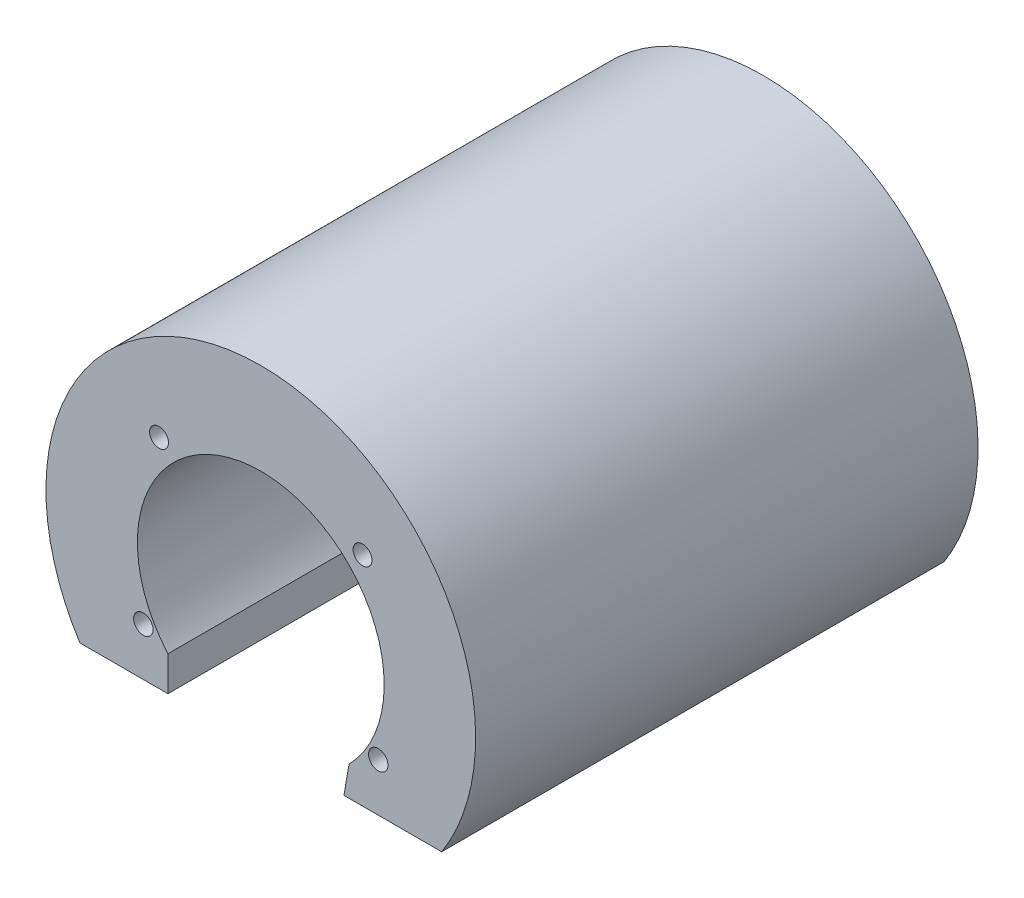
SolidWorks part; units mm, degrees
ref_plane "Front Plane" through (0, 0, 0) normal (0, 0, 1) x (1, 0, 0)
ref_plane "Top Plane" through (0, 0, 0) normal (0, 1, 0) x (1, 0, 0)
ref_plane "Right Plane" through (0, 0, 0) normal (1, 0, 0) x (0, 0, -1)
sketch "Sketch1" plane through (0, 0, 0) normal (0, 0, 1) x (1, 0, 0)
  line L0 (-189.9978, -121.6028) -> (-189.9978, -92.2317)
  line L1 (42.1208, -121.6028) -> (-40.7589, -121.6028)
  line L2 (-189.9978, -121.6028) -> (-264.6407, -121.6028)
  line L5 (-40.7589, -121.6028) -> (-36.4316, -96.4597)
  arc A1 (42.1208, -121.6028) -> (-264.6407, -121.6028) centre (-111.26, -23.3478) ccw
  circle A2 centre (-24.9929, 62.9193) radius 8
  circle A3 centre (-197.527, 62.9193) radius 8
  circle A4 centre (-210.8529, -80.8478) radius 8.25
  circle A5 centre (-11.667, -80.8478) radius 8.25
  arc A6 (-36.4316, -96.4597) -> (-189.9978, -92.2317) centre (-111.26, -23.3478) ccw
  point P18 (-111.26, -23.3478)
extrude "Boss-Extrude1" add sketch "Sketch1" against normal blind 426
